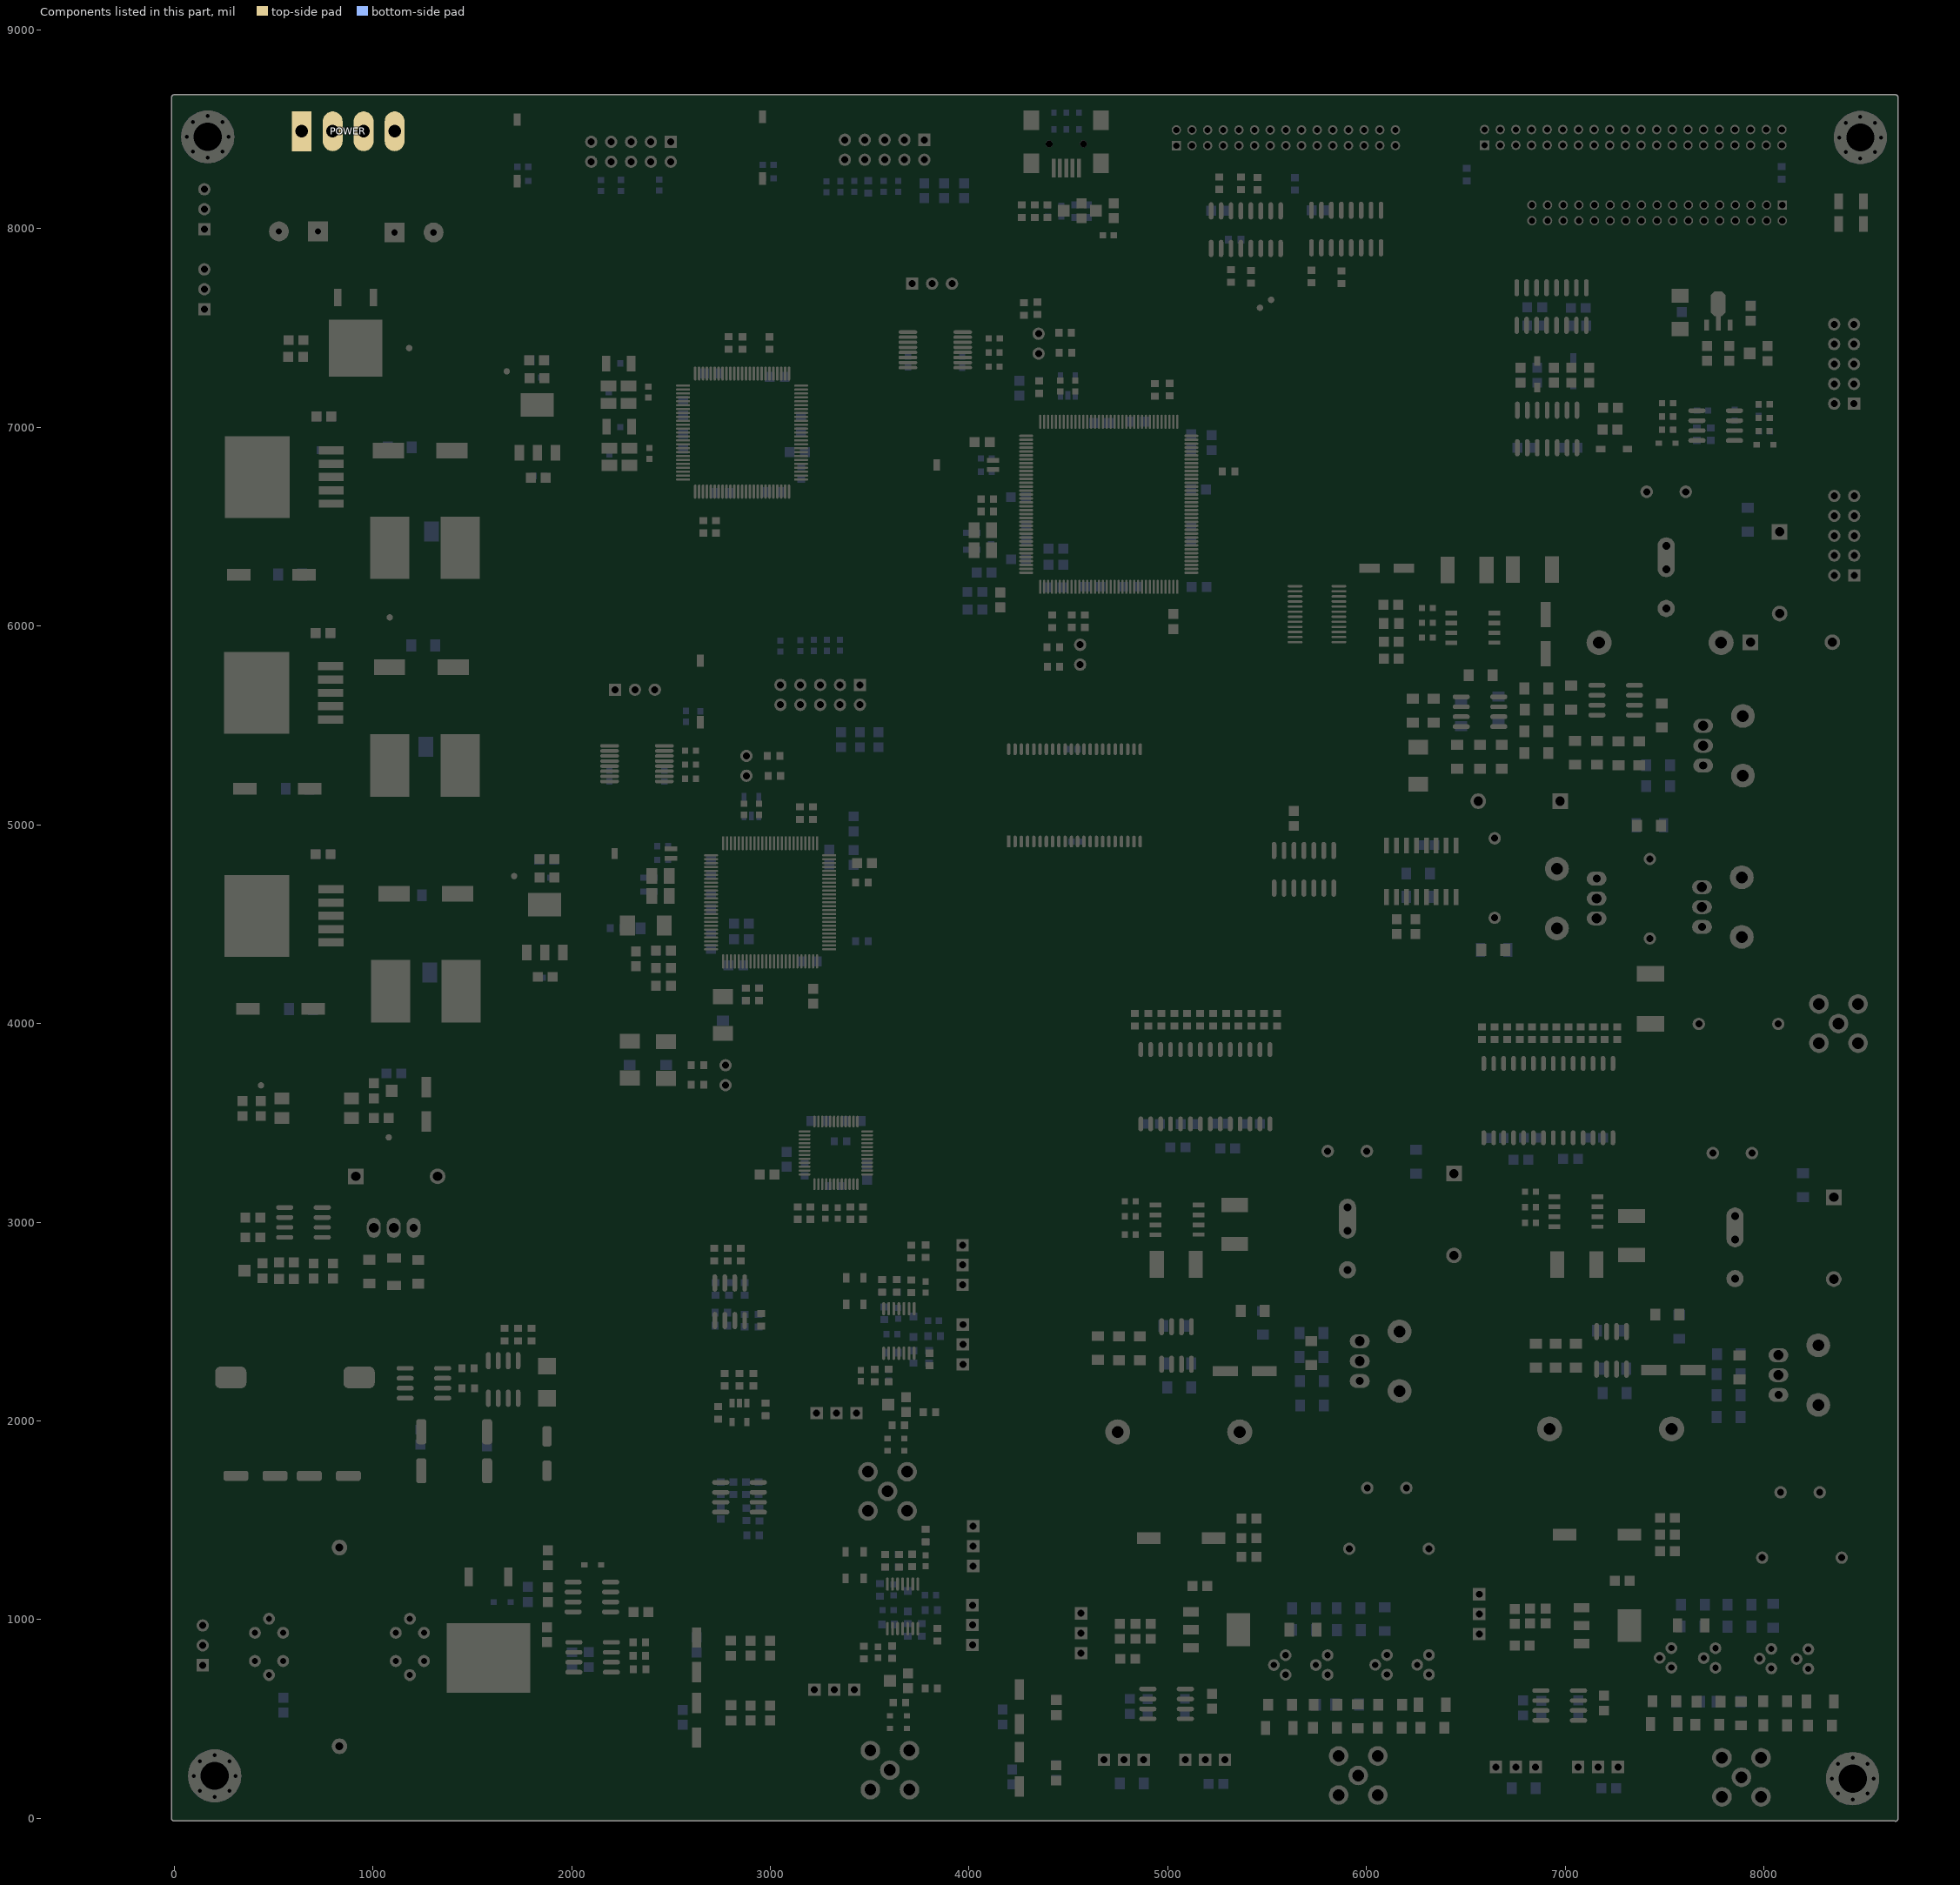
[diagram p0: the components of this part, seen from the top]
# Altium PCB MISC82309.PcbDoc (part 14 of 14)
Units mil, origin at the board's own origin, x right, y up, seen from the top; angles counter-clockwise.
Board outline 8687.03 x 8687.86 mil, 4 copper layers (Top Layer, GND, POWER, Bottom Layer); 747 components, 583 nets, 2530 pads, 1834 vias.

## Other copper (continued)
POWER (plane layer: these items are gaps in the copper):
  region: 7,465 62,520 1234,520 1311,597 1311,1145 1215,1241 58,1241 8,1291 7,1290
  region: 5493,2848 5530,2811 6302,2811 6331,2840 6331,3013 6284,3060 6176,3060 6114,3122 6114,3493 6031,3576 5762,3576 5691,3505 5691,3129 5592,3030 5513,3030 5493,3010
  region: 7439,2794 7453,2780 8251,2780 8267,2796 8267,2971 8246,2992 8097,2992 8046,3043 8046,3498 7983,3561 7669,3561 7630,3522 7630,3000 7598,2968 7450,2968 7439,2957
  region: 7098,6165 7112,6151 7905,6151 7919,6165 7919,6454 7902,6471 7150,6471 7098,6419
  region: 7229,6478 7301,6550 7301,6760 7417,6876 7608,6876 7711,6773 7711,6493 7739,6465 7715,6441 7266,6441
  lines w25: -5,3341 584,3341 663,3262 663,2411 999,2075 1225,2075 1292,2008 1292,1811 ; -2,6579 874,6579 ; 1010,3260 1126,3260 ; 1120,3261 1473,3261 ; 1286,6168 1286,4026 1006,3746 1006,2707 1250,2463 1379,2463 1743,2099 1743,1865 2070,1538 2070,838 2070,800 2071,800 2292,579 3277,579 ; 1290,6171 876,6585 876,6874 987,6985 1418,6985 1560,7127 1624,7127 2014,7127 2097,7044 2097,6787 2313,6571 3077,6571 3245,6739 3245,7309 2696,7858 2696,8391 2868,8563 8056,8563 8293,8326 8528,8091 8528,7702 8494,7668 8494,6552 8292,6350 8292,6241 ; 1293,1830 1293,1803 1593,1503 1594,1503 ; 1418,1680 1704,1394 1704,578 1907,375 6142,375 6158,359 ; 1487,3247 1473,3261 ; 1611,8673 1614,8670 ; 2285,1474 2285,2449 1473,3261 ; 2285,1559 2285,1469 2611,1143 ; 2612,1141 3138,1141 3230,1233 3230,1463 2760,1933 2760,2072 3428,2740 3784,2740 3815,2771 3815,2853 3765,2903 2394,2903 1769,3528 1769,3833 2062,4126 2062,4328 1940,4450 1845,4450 1664,4631 1664,4988 1881,5205 1881,6037 2015,6171 3375,6171 ; 2952,3202 2952,3130 3077,3005 3516,3005 3690,3179 3690,3336 3524,3502 3320,3502 3292,3474 3292,3379 3331,3340 3429,3340 3468,3301 3468,3248 3422,3202 3238,3202 3181,3259 3010,3259 2953,3202 ; 3135,1142 3138,1142 3383,897 7212,897 7765,1450 7765,2069 7728,2106 5214,2106 4805,2515 4805,3853 5294,4342 6903,4342 6952,4391 6952,5834 6777,6009 6745,6009 ; 3274,578 6406,578 6486,498 6486,381 ; 3378,6171 3792,6585 3792,7212 3719,7285 3719,7712 3469,7962 3174,7962 2991,8145 2991,8248 3033,8290 3134,8290 3201,8223 4115,8223 4252,8086 ; 4253,8085 4253,8084 4417,7920 5187,7920 5736,7371 5736,6237 5736,5101 ; 5730,5098 5598,4966 5533,4966 5474,4907 5474,4810 5525,4759 6081,4759 6236,4914 6360,4914 6387,4941 6387,4994 6293,5088 6118,5088 6057,5149 6057,5150 ; 6058,5150 6058,6483 6504,6929 7172,6929 7364,7121 7364,7123 7364,7689 7469,7794 8028,7794 8060,7826 8060,7931 8033,7958 6818,7958 6760,8016 6760,8561 ; 6147,370 6282,235 6439,235 6486,282 6486,374 ; 6490,376 6491,375 7512,375 8066,929 8066,2566 7728,2904 5549,2904 5364,3089 5364,3594 5541,3771 7063,3771 7394,4102 7394,5662 ; 6756,6009 6627,6009 6555,6081 6555,6284 6742,6471 6857,6471 ; 6856,6471 7914,6471 8063,6620 8063,7511 8293,7741 8293,8324 ; 6958,5827 7230,5827 7393,5664 7393,5623 ; 8293,6244 8359,6178 8669,6178